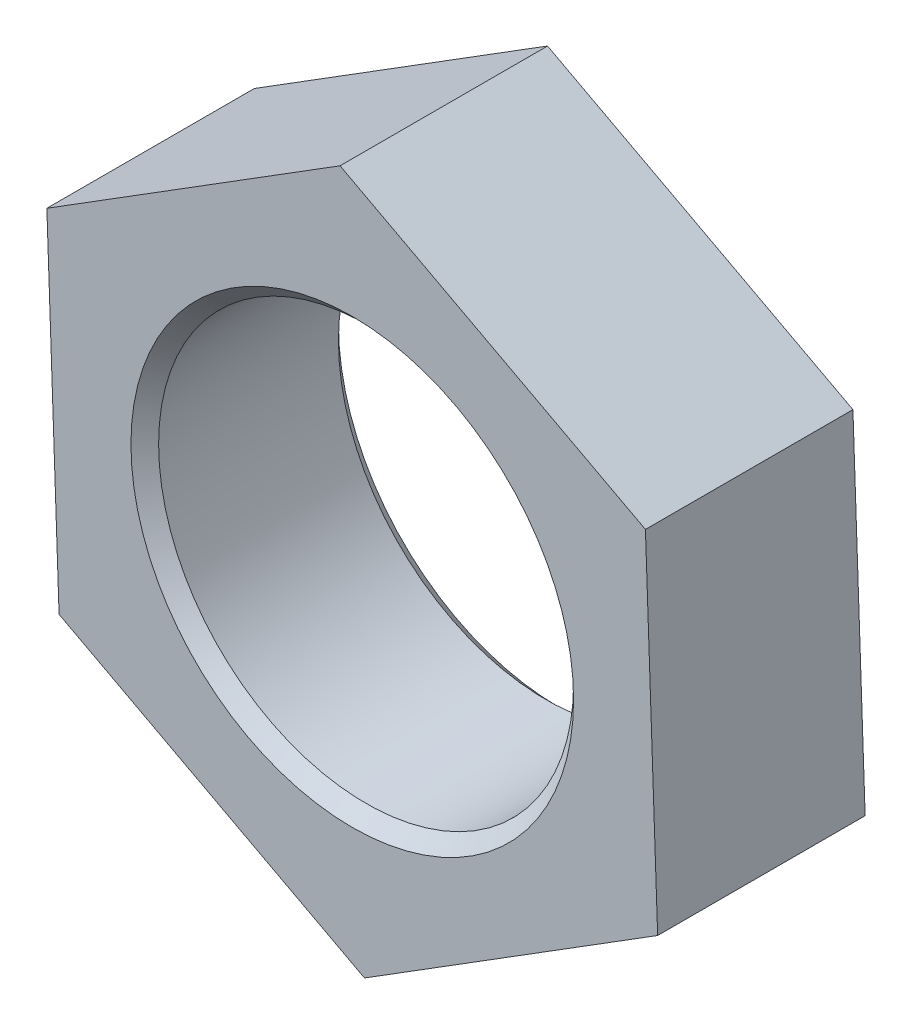
from build123d import *

# Parameters (mm, degrees)
SKETCH1_R           = 15
BOSS_EXTRUDE1_DEPTH = 15
CHAMFER1_SIZE       = 1


with BuildPart() as part:
    # Sketch1 → Boss-Extrude1 (new body)
    with BuildSketch(Plane.XY):
        Polygon((22.078741188, -11.727283895), (21.195496365, 13.257108805), (-0.883244823, 24.9843927), (-22.078741188, 11.727283895), (-21.195496365, -13.257108805), (0.883244823, -24.9843927), align=None)
        Circle(SKETCH1_R, mode=Mode.SUBTRACT)
    extrude(amount=BOSS_EXTRUDE1_DEPTH)

    # Chamfer1
    chamfer1_edges = [part.edges().sort_by_distance(p)[0] for p in [
        (-15, 0, 0),
        (-15, 0, 15),
    ]]
    chamfer(chamfer1_edges, length=CHAMFER1_SIZE)


solid = part.part
